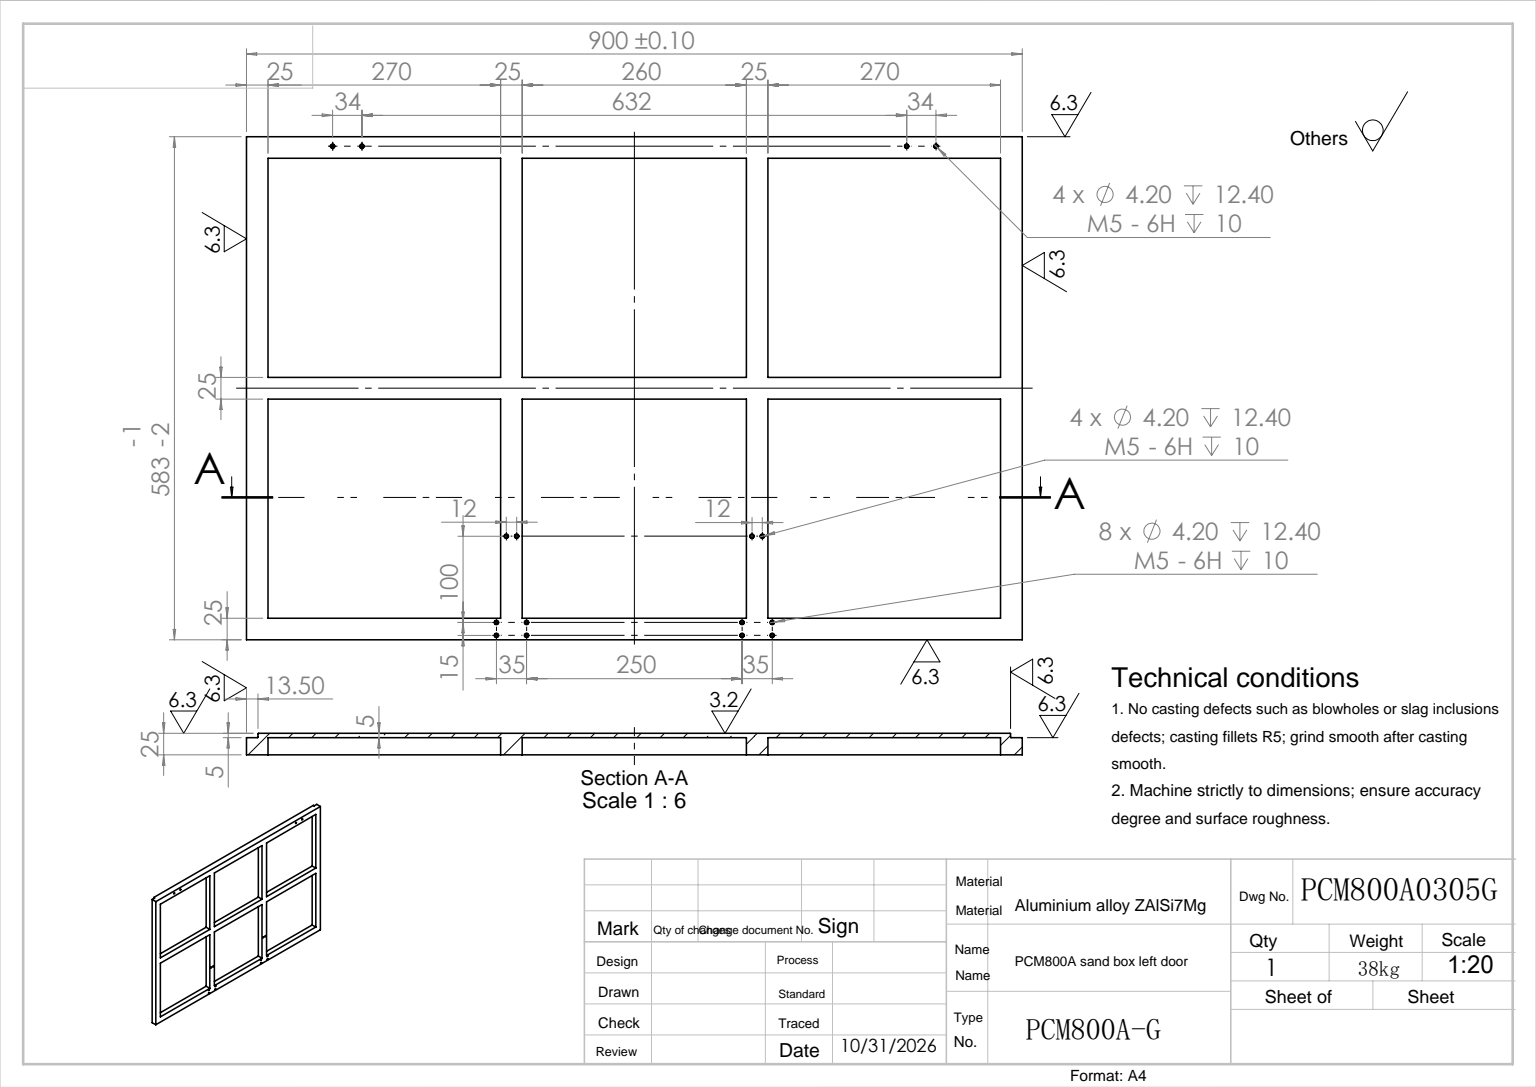
SolidWorks part; units mm, degrees
ref_plane "前视" through (0, 0, 0) normal (0, 0, 1) x (1, 0, 0)
ref_plane "上视" through (0, 0, 0) normal (0, 1, 0) x (1, 0, 0)
ref_plane "右视" through (0, 0, 0) normal (1, 0, 0) x (0, 0, -1)
sketch "草图1" plane through (0, 0, 0) normal (1, 0, 0) x (0, 0, -1)
  line L1 (0, 0) -> (900, 0)
  line L2 (0, 0) -> (0, 583)
  line L3 (0, 583) -> (900, 583)
  line L4 (900, 0) -> (900, 583)
  dimension "D1" = 583
  dimension "D2" = 900
extrude "拉伸1" add sketch "草图1" along normal blind 5
sketch "草图2" plane through (5, 0, 0) normal (1, 0, 0) x (0, 0, -1)
  line L0 (0, 0) -> (900, 0) construction
  line L1 (0, 583) -> (25, 583)
  line L2 (0, 583) -> (0, 0)
  line L3 (0, 0) -> (25, 0)
  line L4 (25, 583) -> (25, 0)
  line L6 (900, 583) -> (875, 583)
  line L7 (900, 583) -> (900, 0)
  line L8 (900, 0) -> (875, 0)
  line L9 (875, 583) -> (875, 0)
  dimension "D1" = 25
  dimension "D2" = 25
extrude "拉伸2" add sketch "草图2" along normal blind 20
sketch "草图3" plane through (5, 0, 0) normal (1, 0, 0) x (0, 0, -1)
  line L0 (875, 583) -> (875, 0) construction
  line L1 (25, 583) -> (875, 583)
  line L2 (25, 583) -> (25, 558)
  line L3 (25, 558) -> (875, 558)
  line L4 (875, 583) -> (875, 558)
  line L5 (875, 583) -> (875, 0) construction
  line L6 (25, 0) -> (875, 0)
  line L7 (25, 0) -> (25, 25)
  line L8 (25, 25) -> (875, 25)
  line L9 (875, 0) -> (875, 25)
  dimension "D1" = 25
  dimension "D2" = 25
extrude "拉伸3" add sketch "草图3" along normal blind 20
sketch "草图4" plane through (5, 0, 0) normal (1, 0, 0) x (0, 0, -1)
  line L0 (25, 25) -> (25, 558) construction
  line L1 (25, 304) -> (875, 304)
  line L2 (25, 304) -> (25, 279)
  line L3 (25, 279) -> (875, 279)
  line L4 (875, 304) -> (875, 279)
  line L5 (875, 558) -> (875, 25) construction
  line L6 (875, 25) -> (25, 25) construction
  dimension "D1" = 25
  dimension "D2" = 254
extrude "拉伸4" add sketch "草图4" along normal blind 20
sketch "草图5" plane through (5, 0, 0) normal (1, 0, 0) x (0, 0, -1)
  line L0 (25, 558) -> (875, 558) construction
  line L1 (295, 558) -> (320, 558)
  line L2 (295, 558) -> (295, 25)
  line L3 (295, 25) -> (320, 25)
  line L4 (320, 558) -> (320, 25)
  line L5 (875, 25) -> (25, 25) construction
  line L6 (25, 558) -> (875, 558) construction
  line L7 (580, 558) -> (605, 558)
  line L8 (580, 558) -> (580, 25)
  line L9 (580, 25) -> (605, 25)
  line L10 (605, 558) -> (605, 25)
  line L11 (25, 304) -> (25, 558) construction
  line L12 (875, 558) -> (875, 304) construction
  dimension "D1" = 25
  dimension "D2" = 25
  dimension "D3" = 270
  dimension "D4" = 270
extrude "拉伸5" add sketch "草图5" along normal blind 20
sketch "草图6" plane through (0, 583, 0) normal (0, 1, 0) x (-1, 0, 0)
  line L1 (0, 0) -> (-5, 0)
  line L2 (0, 0) -> (0, -13.5)
  line L3 (0, -13.5) -> (-5, -13.5)
  line L4 (-5, 0) -> (-5, -13.5)
  dimension "D1" = 5
  dimension "D2" = 13.5
extrude "切除-拉伸1" cut sketch "草图6" against normal through all
chamfer "倒角1" distance 0.5 angle 45 2 edges at (0, 291.5, -13.5) (5, 291.5, -13.5)
sketch "草图7" plane through (0, 583, 0) normal (0, 1, 0) x (-1, 0, 0)
  line L1 (0, -900) -> (-5, -900)
  line L2 (0, -900) -> (0, -886.5)
  line L3 (0, -886.5) -> (-5, -886.5)
  line L4 (-5, -900) -> (-5, -886.5)
  dimension "D1" = 5
  dimension "D2" = 13.5
extrude "切除-拉伸2" cut sketch "草图7" against normal through all
chamfer "倒角2" distance 0.5 angle 45 2 edges at (5, 291.5, -886.5) (0, 291.5, -886.5)
hole_wizard "M5 螺纹孔1" positions "3D草图1" profile "草图8" tap size "M5" standard "GB"
sketch3d "3D草图1"
  line L1 (25, 583, 0) -> (25, 0, 0) construction
  line L2 (25, 0, 0) -> (25, 0, -900) construction
  point P0 (25, 5, -290)
  dimension "D1" = 5
  dimension "D2" = 290
sketch "草图8" plane through (25, 5, -290) normal (0, 1, 0) x (0, 0, -1)
  line L0 (0, 0) -> (0, 13.6618)
  line L1 (0, 13.6618) -> (2.1, 12.4)
  line L2 (2.1, 12.4) -> (2.1, 10)
  line L3 (2.1, 10) -> (2.5, 10)
  line L4 (2.5, 10) -> (2.5, 0)
  line L5 (2.5, 0) -> (0, 0)
  line L10 (0, 13.6618) -> (-2.1, 12.4) construction
  line L11 (0, -6.35) -> (0, 107.95) construction
  dimension "螺纹孔钻头直径" = 4.2
  dimension "螺纹孔钻头深度" = 12.4
  dimension "螺纹主直径" = 5
  dimension "螺纹深度" = 10
  dimension "导头角度" = 118
pattern_linear "阵列(线性)1" count 2 spacing 35 along (0, 0, -1) count 2 spacing 15 along (0, 1, 0) of "M5 螺纹孔1"
hole_wizard "M5 螺纹孔2" positions "3D草图2" profile "草图9" tap size "M5" standard "GB"
sketch3d "3D草图2"
  line L0 (25, 558, -295) -> (25, 304, -295) construction
  line L2 (25, 0, 0) -> (25, 0, -900) construction
  point P0 (25, 120, -301.5)
  point P2 (25, 120, -313.5)
  dimension "D1" = 12
  dimension "D2" = 6.5
  dimension "D3" = 120
  dimension "D4" = 120
sketch "草图9" plane through (25, 120, -301.5) normal (0, 1, 0) x (0, 0, -1)
  line L0 (0, 0) -> (0, 13.6618)
  line L1 (0, 13.6618) -> (2.1, 12.4)
  line L2 (2.1, 12.4) -> (2.1, 10)
  line L3 (2.1, 10) -> (2.5, 10)
  line L4 (2.5, 10) -> (2.5, 0)
  line L5 (2.5, 0) -> (0, 0)
  line L10 (0, 13.6618) -> (-2.1, 12.4) construction
  line L11 (0, -6.35) -> (0, 107.95) construction
  dimension "螺纹孔钻头直径" = 4.2
  dimension "螺纹孔钻头深度" = 12.4
  dimension "螺纹主直径" = 5
  dimension "螺纹深度" = 10
  dimension "导头角度" = 118
pattern_linear "阵列(线性)2" count 2 spacing 285 along (0, 0, -1) of "M5 螺纹孔2", "阵列(线性)1", "M5 螺纹孔1"
hole_wizard "M5 螺纹孔3" positions "3D草图3" profile "草图10" tap size "M5" standard "GB"
sketch3d "3D草图3"
  line L0 (25, 583, -900) -> (25, 583, 0) construction
  line L1 (25, 583, 0) -> (25, 0, 0) construction
  point P0 (25, 572, -100)
  point P2 (25, 572, -134)
  dimension "D1" = 34
  dimension "D2" = 11
  dimension "D3" = 11
  dimension "D4" = 100
sketch "草图10" plane through (25, 572, -100) normal (0, 1, 0) x (0, 0, -1)
  line L0 (0, 0) -> (0, 13.6618)
  line L1 (0, 13.6618) -> (2.1, 12.4)
  line L2 (2.1, 12.4) -> (2.1, 10)
  line L3 (2.1, 10) -> (2.5, 10)
  line L4 (2.5, 10) -> (2.5, 0)
  line L5 (2.5, 0) -> (0, 0)
  line L10 (0, 13.6618) -> (-2.1, 12.4) construction
  line L11 (0, -6.35) -> (0, 107.95) construction
  dimension "螺纹孔钻头直径" = 4.2
  dimension "螺纹孔钻头深度" = 12.4
  dimension "螺纹主直径" = 5
  dimension "螺纹深度" = 10
  dimension "导头角度" = 118
pattern_linear "阵列(线性)3" count 2 spacing 666 along (0, 0, -1) of "M5 螺纹孔3"
